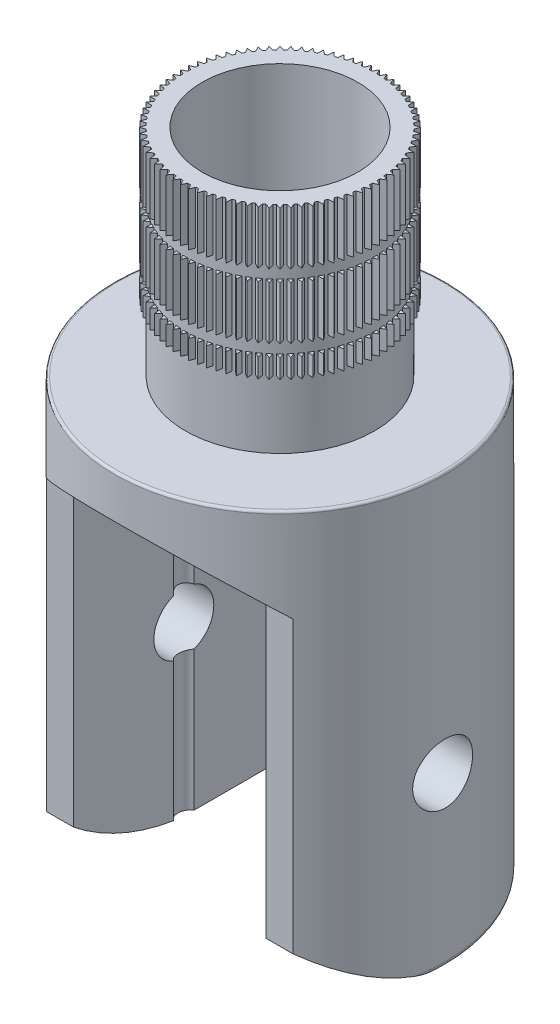
from build123d import *

# Parameters (mm, degrees)
SKETCH3_R               = 3.25
CUT_EXTRUDE1_DEPTH      = 8
CUT_EXTRUDE3_DEPTH      = 7.5
SKETCH4_W               = 8.025
SKETCH4_H               = 11.368420423
CUT_EXTRUDE2_DEPTH      = 14
CUT_EXTRUDE6_DEPTH      = 14
SKETCH9_R               = 1.25
CUT_EXTRUDE7_DEPTH      = 4.9
CUT_EXTRUDE8_DEPTH      = 10
CUT_EXTRUDE8_DEPTH_BACK = 10
SKETCH10_R              = 1.25
FILLET1_R               = 0.2
BOSS_EXTRUDE1_DEPTH     = 6.2
CIRPATTERN1_COUNT       = 80
SKETCH12_W              = 0.2
SKETCH12_H              = 0.5
FILLET2_R               = 0.1


with BuildPart() as part:
    # Sketch1 → Revolve1 (revolve)
    with BuildSketch(Plane.XY):
        Polygon((0, 0), (-6.9, 0), (-6.9, 17.9), (-3.95, 17.9), (-3.95, 26.9), (0, 26.9), align=None)
    revolve(axis=Axis((0, 5.683923158, 0), (0, -1, 0)))

    # Sketch3 → Cut-Extrude1 (cut)
    with BuildSketch(Plane(origin=(0, 26.9, 0), x_dir=(1, 0, 0), z_dir=(0, 1, 0))):
        with Locations(Location((0, 0, 0), (0, 0, 270))):
            Circle(SKETCH3_R)
    extrude(amount=-CUT_EXTRUDE1_DEPTH, mode=Mode.SUBTRACT)

    # Sketch5 → Cut-Extrude3 (cut, symmetric)
    with BuildSketch(Plane(origin=(0, 0, 0), x_dir=(0, 0, -1), z_dir=(1, 0, 0))):
        with BuildLine():
            Line((-6.9, 16.1), (-4.6, 14))
            Line((-4.6, 14), (-4.6, 1.9))
            ThreePointArc((-4.6, 1.9), (-2.481365765, 0.638870557), (-0.1, 0))
            Line((-0.1, 0), (-6.9, 0))
            Line((-6.9, 0), (-6.9, 16.1))
        make_face()
    extrude(amount=CUT_EXTRUDE3_DEPTH, both=True, mode=Mode.SUBTRACT)

    # Sketch4 → Cut-Extrude2 (cut)
    with BuildSketch(Plane.XZ):
        with Locations((0, 1.684210212)):
            Rectangle(SKETCH4_W, SKETCH4_H)
    extrude(amount=-CUT_EXTRUDE2_DEPTH, mode=Mode.SUBTRACT)

    # Sketch8 → Cut-Extrude6 (cut)
    with BuildSketch(Plane.XZ):
        with BuildLine():
            Line((-4.0125, 0.423313987), (-4.0125, -0.423313987))
            ThreePointArc((-4.0125, -0.423313987), (-4.246407407, 0), (-4.0125, 0.423313987))
        make_face()
        with BuildLine():
            Line((4.0125, 0.423313987), (4.0125, -0.423313987))
            ThreePointArc((4.0125, -0.423313987), (4.246407407, 0), (4.0125, 0.423313987))
        make_face()
    extrude(amount=-CUT_EXTRUDE6_DEPTH, mode=Mode.SUBTRACT)

    # Sketch9 → Cut-Extrude7 (cut)
    with BuildSketch(Plane(origin=(0, 18.9, 0), x_dir=(1, 0, 0), z_dir=(0, 1, 0))):
        with Locations(Location((0, 0, 0), (0, 0, 270))):
            Circle(SKETCH9_R)
    extrude(amount=-CUT_EXTRUDE7_DEPTH, mode=Mode.SUBTRACT)

    # Sketch10 → Cut-Extrude8 (cut, two sides: drawn at the far end of the back side and taken through both)
    with BuildSketch(Plane(origin=(0, 0, 0), x_dir=(0, 0, -1), z_dir=(1, 0, 0)).offset(-CUT_EXTRUDE8_DEPTH_BACK)):
        with Locations(Location((0, 7, 0), (0, 0, 180))):
            Circle(SKETCH10_R)
    extrude(amount=CUT_EXTRUDE8_DEPTH + CUT_EXTRUDE8_DEPTH_BACK, mode=Mode.SUBTRACT)

    # Fillet1
    fillet1_edges = [part.edges().sort_by_distance(p)[0] for p in [
        (0.050001313, 0, -6.899818829),
    ]]
    fillet(fillet1_edges, radius=FILLET1_R)

    # Sketch11 → Boss-Extrude1 (add)
    with BuildSketch(Plane(origin=(0, 26.9, 0), x_dir=(1, 0, 0), z_dir=(0, 1, 0))):
        with BuildLine():
            Line((-0.1, 3.948733974), (0, 4.15))
            Line((0, 4.15), (0.1, 3.948733974))
            ThreePointArc((0.1, 3.948733974), (0, 3.95), (-0.1, 3.948733974))
        make_face()
    boss_extrude1 = extrude(amount=-BOSS_EXTRUDE1_DEPTH)

    # CirPattern1: Boss-Extrude1 ×80 about axis
    cirpattern1_axis = Axis((0, 0, 0), (0, 1, 0))
    for i in range(1, CIRPATTERN1_COUNT):
        add(boss_extrude1.rotate(cirpattern1_axis, i * 360 / CIRPATTERN1_COUNT))

    # Sketch12 → Cut-Revolve1 (revolve, cut)
    with BuildSketch(Plane(origin=(0, 0, 0), x_dir=(0, 0, -1), z_dir=(1, 0, 0)), mode=Mode.PRIVATE) as cut_revolve1_sk:
        with Locations((-4.05, 24.45)):
            Rectangle(SKETCH12_W, SKETCH12_H)
        with Locations((-4.05, 21.75)):
            Rectangle(SKETCH12_W, SKETCH12_H)
    revolve(cut_revolve1_sk.sketch.rotate(Axis((0, 8.707611845, 0), (0, 1, 0)), 270), axis=Axis((0, 8.707611845, 0), (0, 1, 0)), mode=Mode.SUBTRACT)

    # Fillet2
    fillet2_edges = [part.edges().sort_by_distance(p)[0] for p in [
        (6.9, 17.9, 0),
    ]]
    fillet(fillet2_edges, radius=FILLET2_R)


solid = part.part
